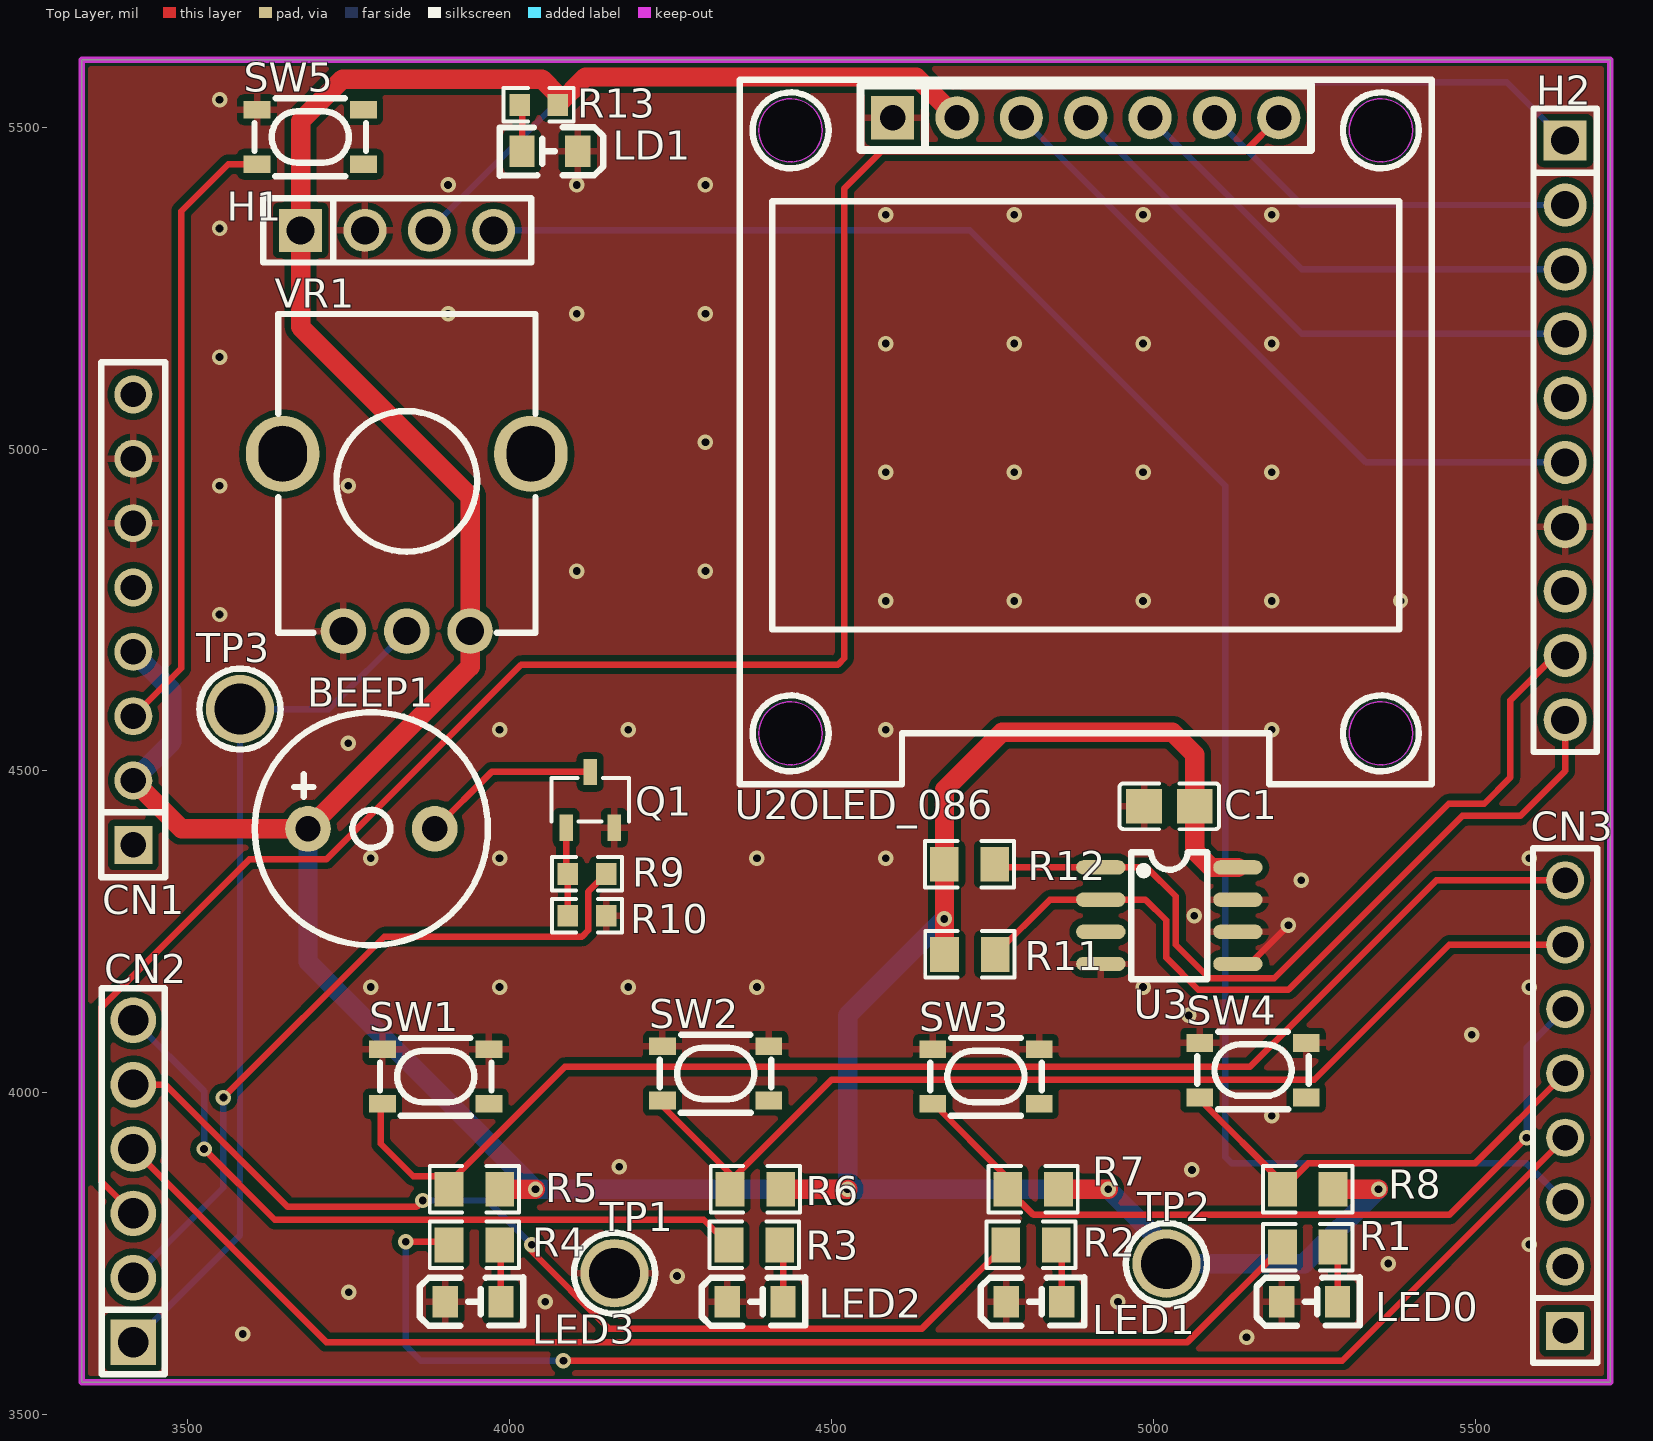
[diagram p0: Top Layer view]
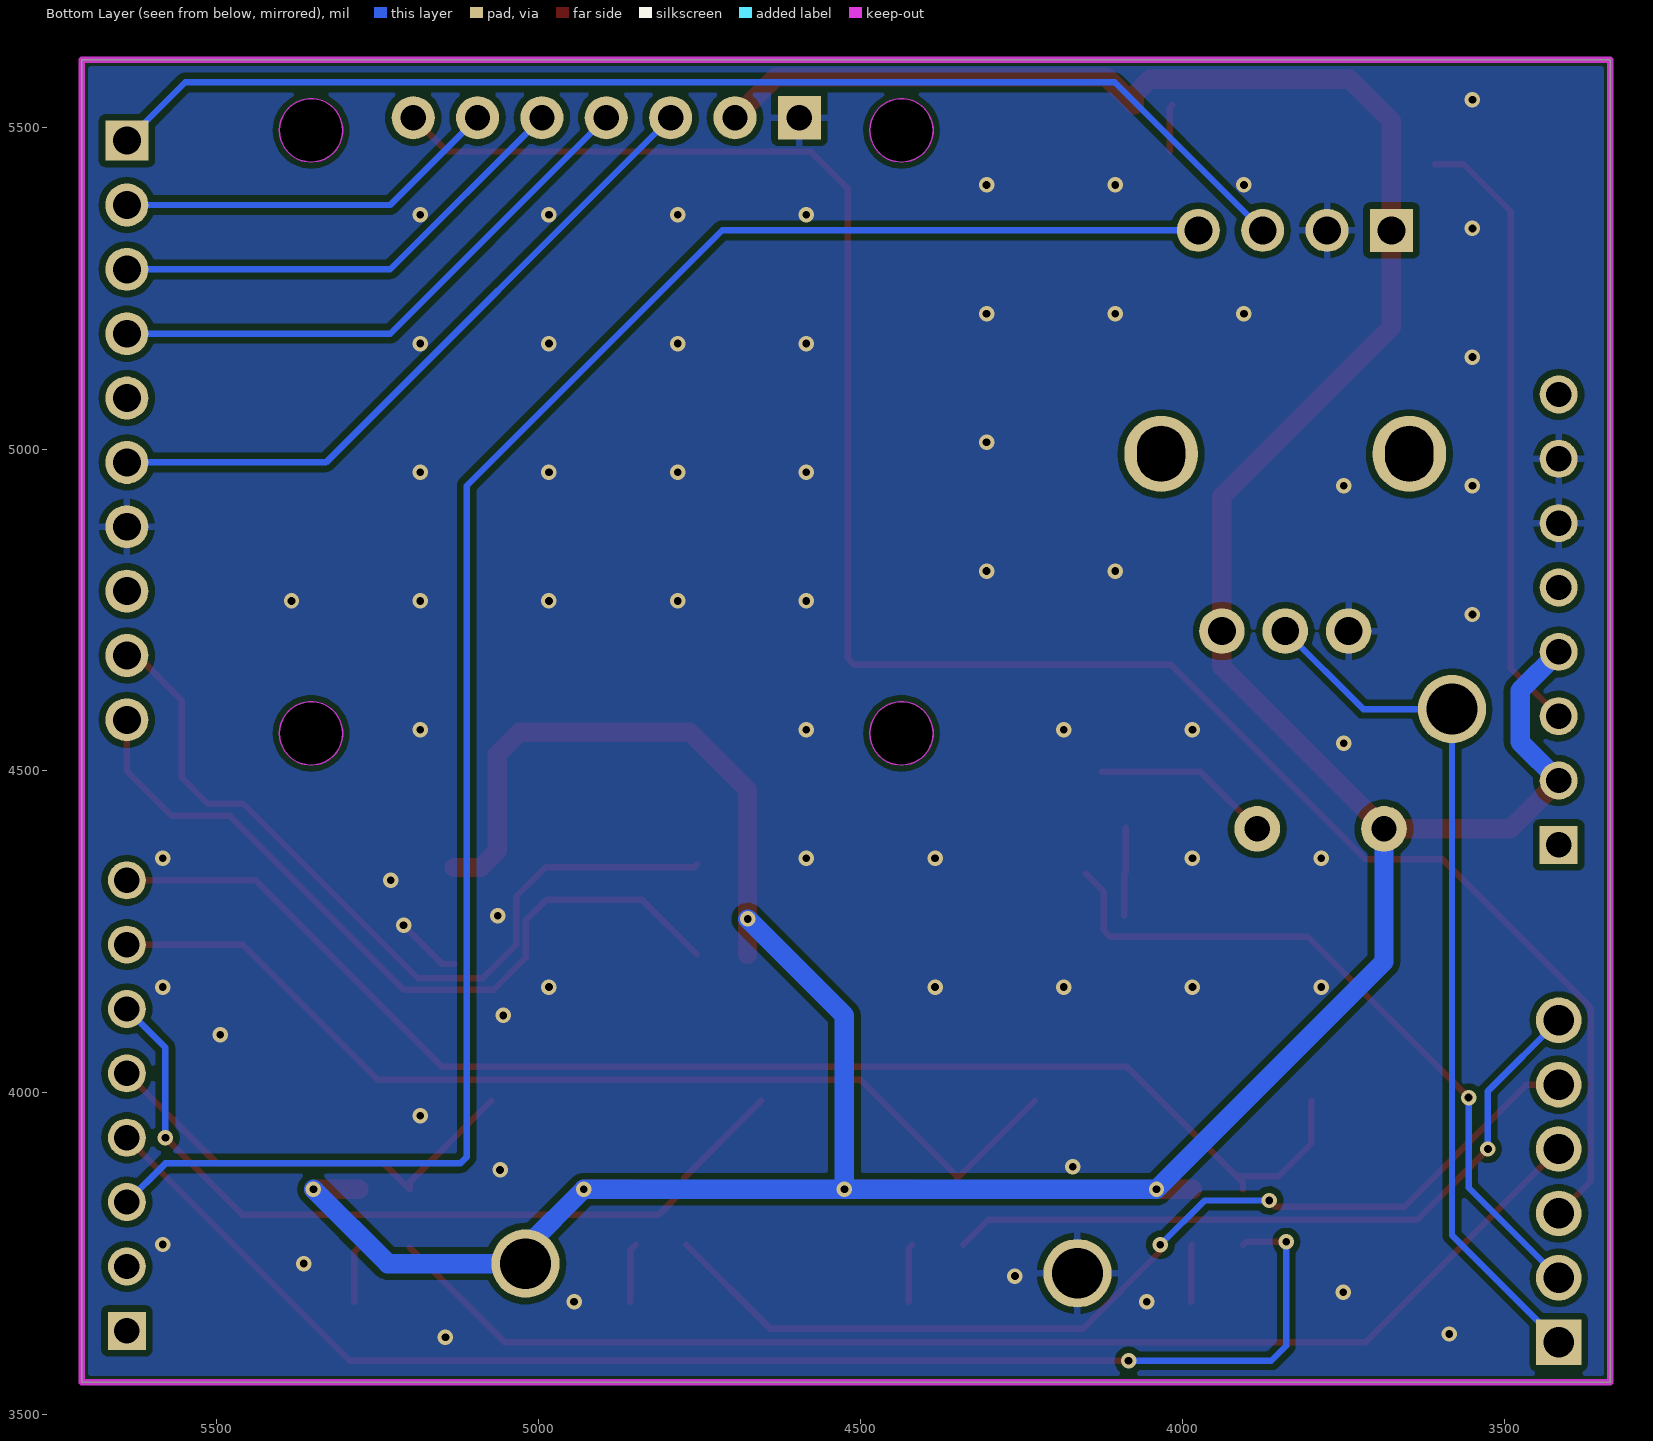
[diagram p1: Bottom Layer view, seen from below]
# Altium PCB MISC51904.pcbdoc
Units mil, origin at the board's own origin, x right, y up, seen from the top; angles counter-clockwise.
Board outline 2375 x 2055 mil, 2 copper layers (Top Layer, Bottom Layer), stack 62.206 mil thick; 37 components, 32 nets, 122 pads, 76 vias.

## Layer stack, top to bottom
Top Solder Mask Layer: solder mask 0.394, Dk 3.3
Top Layer: signal copper 1.379
Dielectric1: surface 59.449, FR4, Dk 4.5
Bottom Layer: signal copper 1.378
Bottom Solder Mask Layer: solder mask 0.394, Dk 3.3

## Board outline
3335,5605 3335,3550 5710,3550 5710,5605

## Design rules (kind name [scope] priority, off if disabled: settings)
BoardOutlineClearance copperThickness2oz_1 [All] p2 off: genericclearance=7.99 ignorepadtopadclearanceinfootprint=FALSE except(0: Arc-SplitContinuation Track-SplitContinuation SMDPad-SplitContinuation THPad-SplitContinuation Via-SplitContinuation Fill-SplitContinuation Region-SplitContinuation Poly-SplitContinuation Text-SplitContinuation Hole-SplitContinuation; 5.98: Arc-CutoutEdge SMDPad-CutoutEdge THPad-CutoutEdge Via-CutoutEdge Fill-CutoutEdge Region-CutoutEdge Text-CutoutEdge; 6.93: Hole-OutlineEdge Hole-CutoutEdge; 10: Poly-OutlineEdge Poly-CutoutEdge; 11.81: Arc-OutlineEdge Track-OutlineEdge SMDPad-OutlineEdge THPad-OutlineEdge Via-OutlineEdge Fill-OutlineEdge Region-OutlineEdge Text-OutlineEdge Track-CutoutEdge)
BoardOutlineClearance copperThickness1oz_1 [All] p4: genericclearance=4.02 ignorepadtopadclearanceinfootprint=FALSE except(0: Arc-SplitContinuation Track-SplitContinuation SMDPad-SplitContinuation THPad-SplitContinuation Via-SplitContinuation Fill-SplitContinuation Region-SplitContinuation Poly-SplitContinuation Text-SplitContinuation Hole-SplitContinuation; 6: SMDPad-CutoutEdge THPad-CutoutEdge Via-CutoutEdge Fill-CutoutEdge Region-CutoutEdge Text-CutoutEdge; 6.93: Hole-OutlineEdge Hole-CutoutEdge; 10: Poly-OutlineEdge Poly-CutoutEdge; 11.8: Arc-OutlineEdge Track-OutlineEdge SMDPad-OutlineEdge THPad-OutlineEdge Via-OutlineEdge Fill-OutlineEdge Region-OutlineEdge Text-OutlineEdge; 11.81: Arc-CutoutEdge Track-CutoutEdge)
Clearance copperThickness2oz [All] p1 off: gap=7.99 ignorepadtopadclearanceinfootprint=FALSE except(5.98: SMDPad-Track SMDPad-SMDPad THPad-Track SMDPad-THPad THPad-THPad Track-Via SMDPad-Via THPad-Via Via-Via Fill-Track Region-Track Fill-SMDPad Region-SMDPad Fill-THPad Region-THPad Fill-Via Region-Via Fill-Fill Fill-Region Region-Region Arc-Track Arc-SMDPad Arc-THPad Arc-Via Fill-Arc Region-Arc Arc-Arc Text-Track SMDPad-Text Text-THPad Text-Via Fill-Text Region-Text Arc-Text Text-Text; 6.93: Hole-Track Hole-SMDPad Hole-THPad Hole-Via Fill-Hole Region-Hole Hole-Arc Hole-Text; 10: Poly-Track Poly-SMDPad Poly-THPad Poly-Via Poly-Fill Poly-Region Poly-Poly Poly-Arc Poly-Text Poly-Hole)
Clearance copperThickness1oz [All] p3: gap=4.02 ignorepadtopadclearanceinfootprint=FALSE except(5.98: SMDPad-Track SMDPad-SMDPad THPad-Track SMDPad-THPad THPad-THPad Track-Via SMDPad-Via THPad-Via Via-Via Fill-Track Region-Track Fill-SMDPad Region-SMDPad Fill-THPad Region-THPad Fill-Via Region-Via Fill-Fill Fill-Region Region-Region; 6: Arc-Track Arc-SMDPad Arc-THPad Arc-Via Fill-Arc Region-Arc Arc-Arc Text-Track SMDPad-Text Text-THPad Text-Via Fill-Text Region-Text Arc-Text Text-Text; 6.93: Hole-Track Hole-SMDPad Hole-THPad Hole-Via Fill-Hole Region-Hole Hole-Arc Hole-Text; 10: Poly-Track Poly-SMDPad Poly-THPad Poly-Via Poly-Fill Poly-Region Poly-Poly Poly-Arc Poly-Text Poly-Hole)
DiffPairsRouting differentialPair [All] p1: maxlimit=6 minlimit=6 mostfreqgap=6 toplayer_minwidth=5 toplayer_prefwidth=10 toplayer_maxwidth=100 toplayer_mingap=6 toplayer_prefgap=6 toplayer_maxgap=6 bottomlayer_minwidth=5 bottomlayer_prefwidth=10 bottomlayer_maxwidth=100 bottomlayer_mingap=6 bottomlayer_prefgap=6 bottomlayer_maxgap=6 maxuncoupledlength=10
HoleToHoleClearance otherClearance [All] p1: gap=11.81 allowstackedmicrovias=TRUE
Length netLength [All] p1: minlimit=0 maxlimit=0
MatchedLengths netLengthTolerance [All] p1: tolerance=1000
PasteMaskExpansion pasteMaskExpansion [All] p1: expansion=0
PlaneConnect innerPlane [All] p1: planeconnectstyle=Relief reliefexpansion=20 reliefentries=4 reliefconductorwidth=10 reliefairgap=10
PolygonConnect copperRegion [(InNet('GND'))] p1: connectstyle=Relief reliefconductorwidth=10 reliefentries=4 polygonreliefangle="90 Angle" airgapwidth=10 via.connectstyle=Relief via.reliefconductorwidth=10 via.reliefentries=4 via.polygonreliefangle="90 Angle" via.airgapwidth=10
RoutingVias viaSize [All] p1: holewidth=12.01 width=24.02 viastyle="Through Hole" minholewidth=11.81 minwidth=19.68 maxholewidth=248.03 maxwidth=393.7
SolderMaskExpansion solderMaskExpansion [IsVia] p1: expansion=-1000 istentingtop=TRUE
SolderMaskExpansion solderMaskExpansion [All] p2: expansion=2 istentingtop=FALSE
Width copperThickness2oz_2 [All] p1 off: maxlimit=100 minlimit=8 preferedwidth=10
Width copperThickness1oz_2 [All] p2: maxlimit=100 minlimit=5 preferedwidth=10

## Components (designator, comment, footprint, x,y, rotation, side; value= is the part's Value field where it differs from the comment)
BEEP1 "3kHz" BUZ-TH_BD9.0-P5.00-D0.6-FD 3785,4410 r0 top
C1 "100nF" C0805 5025,4445 r180 top
CN1 "" HDR-TH_8P-P2.54-V-M 3415,4735 r90 top
CN2 "" HDR-TH_6P-P2.54-V-M-1 3415.02,3862.46 r90 top
CN3 "" HDR-TH_8P-P2.54-V-M 5640,3980 r90 top
H1 "" HDR-TH_4P-P2.54-V-F 3825,5340 r0 top
H2 "" HDR-TH_10P-P2.54-V-M-1 5640,5029.37 r270 top
LD1 "NCD0805R1" LED0805-RD 4062.44,5462.83 r180 top
LED0 "" LED_0805 5245,3675 r0 top
LED1 "" LED_0805 4816.67,3675 r0 top
LED2 "" LED_0805 4383.33,3675 r0 top
LED3 "" LED_0805 3945,3675 r0 top
Q1 "S8050 J3Y(RANGE:200-350)" SOT-23-3_L3.0-W1.7-P0.95-LS2.9-BR 4125,4455 r270 top
R1 "4.7K" R0805 5240,3760 r0 top
R2 "4.7K" R0805 4810,3763.48 r0 top
R3 "4.7K" R0805 4380,3763.48 r0 top
R4 "4.7K" R0805 3945,3763.48 r0 top
R5 "4.7kΩ" R0805 3945,3850 r0 top
R6 "4.7kΩ" R0805 4381.67,3850 r0 top
R7 "4.7kΩ" R0805 4813.33,3850 r0 top
R8 "4.7kΩ" R0805 5240,3850 r0 top
R9 "1K" R0603 4120,4340 r0 top
R10 "10K" R0603 4120,4275 r180 top
R11 "4.7kΩ" R0805 4715,4215 r180 top
R12 "4.7kΩ" R0805 4714.45,4354.91 r0 top
R13 "4.7K" R0603 4045,5535 r0 top
SW1 "" Key_SMD_4.2x3.2x2.5 3885,4025 r0 top
SW2 "" Key_SMD_4.2x3.2x2.5 4320,4030 r0 top
SW3 "" Key_SMD_4.2x3.2x2.5 4740,4025 r0 top
SW4 "" Key_SMD_4.2x3.2x2.5 5155,4035 r0 top
SW5 "" Key_SMD_4.2x3.2x2.5 3690,5485 r0 top
TP1 "TP-红色测试点" TESTPOINT-TH_BD3.2 4162.83,3719.39 r0 top
TP2 "TP-红色测试点" TESTPOINT-TH_BD3.2 5020.52,3734.39 r0 top
TP3 "TP-红色测试点" TESTPOINT-TH_BD3.2 3580.83,4596.07 r0 top
U2OLED_086 "0.96寸OLED_7P" OLED-TH_HS96L01W4S03 4895,5515 r0 top
U3 "LM75AD,118" SOIC-8_L5.0-W4.0-P1.27-LS6.0-BL 5025,4275 r270 top
VR1 "10kΩ" RES-ADJ-TH_RK09K1130AJ3 3840,4855 r0 top

## Footprints (in the part's own frame and the unit in brackets; to place one, negate y for a bottom-side part, rotate by r counter-clockwise, add the part's x,y. Pads: shape width x height; smd on the part's side, far side on the other; paste and mask are expansions set on the pad)
BUZ-TH_BD9.0-P5.00-D0.6-FD [mm]
  round 1.8 hole 1 copper offset 0,0: 1(-2.5,0)
  round 1.8 hole 1: 2(2.5,0)
  silkscreen extent -4.6,-4.6 4.6,4.6
C0805 [mm]
  rect 1.41x1.35 smd paste-100 mask+0.051: 1(-1,0) 2(1,0)
  silkscreen extent -1.96,-0.9 1.96,0.9
HDR-TH_4P-P2.54-V-F [mm]
  rect 1.7x1.7 hole 1.1: 1(-3.81,0)
  round 1.7 hole 1.1: 2(-1.27,0) 3(1.27,0) 4(3.81,0)
  silkscreen extent -5.29,-1.27 5.29,1.27
HDR-TH_6P-P2.54-V-M-1 [mm]
  rect 1.8x1.8 hole 1.2: 1(-6.35,0)
  round 1.8 hole 1.2: 2(-3.81,0) 3(-1.27,0) 4(1.27,0) 5(3.81,0) 6(6.35,0)
  silkscreen extent -7.62,-1.25 7.62,1.25
HDR-TH_8P-P2.54-V-M [mm]
  rect 1.5x1.5 hole 1: 1(-8.89,0)
  round 1.5 hole 1: 2(-6.35,0) 3(-3.81,0) 4(-1.27,0) 5(1.27,0) 6(3.81,0) 7(6.35,0) 8(8.89,0)
  silkscreen extent -10.16,-1.27 10.16,1.27
HDR-TH_10P-P2.54-V-M-1 [mm]
  rect 1.575x1.7 hole 1.1: 1(-11.43,0)
  round 1.7 hole 1.1: 2(-8.89,0) 3(-6.35,0) 4(-3.81,0) 5(-1.27,0) 6(1.27,0) 7(3.81,0) 8(6.35,0) 9(8.89,0) 10(11.43,0)
  silkscreen extent -12.7,-1.25 12.7,1.25
Key_SMD_4.2x3.2x2.5 [mil]
  rect 41.3x27.6 smd paste+0 mask+2: 1(-82.7,42.3) 2(82.7,42.3) 3(-82.7,-42.3) 4(82.7,-42.3)
  silkscreen extent -87,-61 87,60
LED0805-RD [mm]
  rect 1x1.25 smd: 1(-1.1,0) 2(1.1,0)
  silkscreen extent -2.1,-0.95 1.98,0.96
LED_0805 [mm]
  rect 1x1.25 smd paste+0 mask+0.051: 1(-1.15,0.005) 2(1.05,0.005)
  silkscreen extent -2.15,-0.94 1.93,0.97
OLED-TH_HS96L01W4S03 [mm]
  rect 1.7x1.7 hole 1: 1(-7.62,0)
  round 1.7 hole 1: 2(-5.08,0) 3(-2.54,0) 4(0,0) 5(2.54,0) 6(5.08,0) 7(7.62,0)
  Board Outline Layer circle w0.003: c11.65,-0.5 r1.25
  Board Outline Layer circle w0.003: c-11.65,-0.5 r1.25
  Board Outline Layer circle w0.003: c-11.65,-24.3 r1.25
  Board Outline Layer circle w0.003: c11.65,-24.3 r1.25
  Board Outline Layer region: 12.9,-0.5 12.776,-1.042 12.429,-1.477 11.928,-1.719 11.372,-1.719 10.871,-1.477 10.524,-1.042 10.4,-0.5 10.4,-0.5 10.524,0.042 10.871,0.477 11.372,0.719 11.928,0.719 12.429,0.477 12.776,0.042 12.9,-0.5
  Board Outline Layer region: 12.9,-0.5 12.89,-0.657 12.861,-0.811 12.812,-0.96 12.745,-1.102 12.661,-1.235 12.561,-1.356 12.447,-1.463 12.32,-1.555 12.182,-1.631 12.036,-1.689 11.884,-1.728 11.728,-1.747 11.571,-1.747 11.416,-1.728 11.264,-1.689 11.118,-1.631 10.98,-1.555 10.853,-1.463 10.739,-1.356 10.639,-1.235 10.555,-1.102 10.488,-0.96 10.439,-0.811 10.41,-0.657 10.4,-0.5 10.41,-0.343 10.439,-0.189 10.488,-0.04 10.555,0.102 10.639,0.235 10.739,0.356 10.853,0.463 10.98,0.556 11.118,0.631 11.264,0.689 11.416,0.728 11.571,0.748 11.728,0.748 11.884,0.728 12.036,0.689 12.182,0.631 12.32,0.556 12.447,0.463 12.561,0.356 12.661,0.235 12.745,0.102 12.812,-0.04 12.861,-0.189 12.89,-0.343
  Board Outline Layer region: -10.4,-0.5 -10.524,-1.042 -10.871,-1.477 -11.372,-1.719 -11.928,-1.719 -12.429,-1.477 -12.776,-1.042 -12.9,-0.5 -12.9,-0.5 -12.776,0.042 -12.429,0.477 -11.928,0.719 -11.372,0.719 -10.871,0.477 -10.524,0.042 -10.4,-0.5
  Board Outline Layer region: -10.4,-0.5 -10.41,-0.657 -10.439,-0.811 -10.488,-0.96 -10.555,-1.102 -10.639,-1.235 -10.739,-1.356 -10.853,-1.463 -10.98,-1.555 -11.118,-1.631 -11.264,-1.689 -11.416,-1.728 -11.571,-1.747 -11.728,-1.747 -11.884,-1.728 -12.036,-1.689 -12.182,-1.631 -12.32,-1.555 -12.447,-1.463 -12.561,-1.356 -12.661,-1.235 -12.745,-1.102 -12.812,-0.96 -12.861,-0.811 -12.89,-0.657 -12.9,-0.5 -12.89,-0.343 -12.861,-0.189 -12.812,-0.04 -12.745,0.102 -12.661,0.235 -12.561,0.356 -12.447,0.463 -12.32,0.556 -12.182,0.631 -12.036,0.689 -11.884,0.728 -11.728,0.748 -11.571,0.748 -11.416,0.728 -11.264,0.689 -11.118,0.631 -10.98,0.556 -10.853,0.463 -10.739,0.356 -10.639,0.235 -10.555,0.102 -10.488,-0.04 -10.439,-0.189 -10.41,-0.343
  Board Outline Layer region: -10.4,-24.3 -10.524,-24.842 -10.871,-25.277 -11.372,-25.519 -11.928,-25.519 -12.429,-25.277 -12.776,-24.842 -12.9,-24.3 -12.9,-24.3 -12.776,-23.758 -12.429,-23.323 -11.928,-23.081 -11.372,-23.081 -10.871,-23.323 -10.524,-23.758 -10.4,-24.3
  Board Outline Layer region: -10.4,-24.3 -10.41,-24.457 -10.439,-24.611 -10.488,-24.76 -10.555,-24.902 -10.639,-25.035 -10.739,-25.156 -10.853,-25.263 -10.98,-25.355 -11.118,-25.431 -11.264,-25.489 -11.416,-25.528 -11.571,-25.547 -11.728,-25.547 -11.884,-25.528 -12.036,-25.489 -12.182,-25.431 -12.32,-25.355 -12.447,-25.263 -12.561,-25.156 -12.661,-25.035 -12.745,-24.902 -12.812,-24.76 -12.861,-24.611 -12.89,-24.457 -12.9,-24.3 -12.89,-24.143 -12.861,-23.989 -12.812,-23.84 -12.745,-23.698 -12.661,-23.565 -12.561,-23.444 -12.447,-23.337 -12.32,-23.245 -12.182,-23.169 -12.036,-23.111 -11.884,-23.072 -11.728,-23.052 -11.571,-23.052 -11.416,-23.072 -11.264,-23.111 -11.118,-23.169 -10.98,-23.245 -10.853,-23.337 -10.739,-23.444 -10.639,-23.565 -10.555,-23.698 -10.488,-23.84 -10.439,-23.989 -10.41,-24.143
  Board Outline Layer region: 12.9,-24.3 12.776,-24.842 12.429,-25.277 11.928,-25.519 11.372,-25.519 10.871,-25.277 10.524,-24.842 10.4,-24.3 10.4,-24.3 10.524,-23.758 10.871,-23.323 11.372,-23.081 11.928,-23.081 12.429,-23.323 12.776,-23.758 12.9,-24.3
  Board Outline Layer region: 12.9,-24.3 12.89,-24.457 12.861,-24.611 12.812,-24.76 12.745,-24.902 12.661,-25.035 12.561,-25.156 12.447,-25.263 12.32,-25.355 12.182,-25.431 12.036,-25.489 11.884,-25.528 11.728,-25.547 11.571,-25.547 11.416,-25.528 11.264,-25.489 11.118,-25.431 10.98,-25.355 10.853,-25.263 10.739,-25.156 10.639,-25.035 10.555,-24.902 10.488,-24.76 10.439,-24.611 10.41,-24.457 10.4,-24.3 10.41,-24.143 10.439,-23.989 10.488,-23.84 10.555,-23.698 10.639,-23.565 10.739,-23.444 10.853,-23.337 10.98,-23.245 11.118,-23.169 11.264,-23.111 11.416,-23.072 11.571,-23.052 11.728,-23.052 11.884,-23.072 12.036,-23.111 12.182,-23.169 12.32,-23.245 12.447,-23.337 12.561,-23.444 12.661,-23.565 12.745,-23.698 12.812,-23.84 12.861,-23.989 12.89,-24.143
  Multi-Layer board cut-out: 12.9,-0.5 12.776,-1.042 12.429,-1.477 11.928,-1.719 11.372,-1.719 10.871,-1.477 10.524,-1.042 10.4,-0.5 10.4,-0.5 10.524,0.042 10.871,0.477 11.372,0.719 11.928,0.719 12.429,0.477 12.776,0.042 12.9,-0.5
  Multi-Layer board cut-out: -10.4,-0.5 -10.524,-1.042 -10.871,-1.477 -11.372,-1.719 -11.928,-1.719 -12.429,-1.477 -12.776,-1.042 -12.9,-0.5 -12.9,-0.5 -12.776,0.042 -12.429,0.477 -11.928,0.719 -11.372,0.719 -10.871,0.477 -10.524,0.042 -10.4,-0.5
  Multi-Layer board cut-out: -10.4,-24.3 -10.524,-24.842 -10.871,-25.277 -11.372,-25.519 -11.928,-25.519 -12.429,-25.277 -12.776,-24.842 -12.9,-24.3 -12.9,-24.3 -12.776,-23.758 -12.429,-23.323 -11.928,-23.081 -11.372,-23.081 -10.871,-23.323 -10.524,-23.758 -10.4,-24.3
  Multi-Layer board cut-out: 12.9,-24.3 12.776,-24.842 12.429,-25.277 11.928,-25.519 11.372,-25.519 10.871,-25.277 10.524,-24.842 10.4,-24.3 10.4,-24.3 10.524,-23.758 10.871,-23.323 11.372,-23.081 11.928,-23.081 12.429,-23.323 12.776,-23.758 12.9,-24.3
  silkscreen extent -13.65,-26.3 13.65,1.5
R0603 [mil]
  rect 31.75x34.02 smd paste-3937.01 mask+2: 1(-29.66,0) 2(29.66,0)
  silkscreen extent -55,-26 55,26
R0805 [mm]
  rect 1.133x1.377 smd paste-100 mask+0.051: 1(-1,0) 2(1,0)
  silkscreen extent -1.76,-0.92 1.76,0.92
RES-ADJ-TH_RK09K1130AJ3 [mm]
  round 1.8 hole 1.1: 1(-2.5,-3.5) 2(0,-3.5) 3(2.5,-3.5)
  oval 2.9x3 hole 1.9 slot 2.2 at 90 deg: 4(-4.9,3.5) 5(4.9,3.5)
  silkscreen extent -5.08,-3.56 5.08,9.02
SOIC-8_L5.0-W4.0-P1.27-LS6.0-BL [mil]
  oval 22.38x76.78 smd: 1(-75,-106.5) 2(-25,-106.5) 3(25,-106.5) 4(75,-106.5) 5(75,106.5) 6(25,106.5) 7(-25,106.5) 8(-75,106.5)
  silkscreen extent -98,-59 98,59
SOT-23-3_L3.0-W1.7-P0.95-LS2.9-BR [mil]
  rect 40.85x20.95 smd: 1(43.36,-37.4) 2(43.36,37.4) 3(-43.36,0)
  silkscreen extent -34,-60 34,60
TESTPOINT-TH_BD3.2 [mm]
  round 2.7 hole 2 paste+0 mask+0.05: 1(0,0)
  silkscreen extent -1.6,-1.6 1.6,1.6

## Via types
v1: diameter 24.02, hole 12, Top Layer to Bottom Layer, 76 vias

## Nets (pads, with @x,y where several pads share a name; then routed paths per layer and width w, separated by ;. In a path a pad name is that pad's centre, name@x,y a point inside that pad or via, vN(x,y) a via of type N, cw(c..) or ccw(c..) an arc to the next point about the centre after c; other vN are vias at no path point)
$1N7: LED0.2 R1.2 | length 87.7
  Top Layer w10: R1.2 5286.34,3753.03 LED0.2
$1N9: LED1.2 R2.2 | length 91.9
  Top Layer w10: R2.2 4858.01,3754.84 LED1.2
$1N10: LED2.2 R3.2 | length 90.5
  Top Layer w10: R3.2 4424.67,3758.18 LED2.2
$1N11: LED3.2 R4.2 | length 89.1
  Top Layer w10: R4.2 3986.34,3761.51 LED3.2
$1N39: BEEP1.2 Q1.3 | length 278.2
  Top Layer w10: BEEP1.2 3971.78,4498.36 Q1.3
$1N40: Q1.1 R9.1 R10.2 | length 137.8
  Top Layer w10: Q1.1 4087.6,4342.74 R9.1 R10.2
$1N62: CN1.3 SW5.3 | length 963.7
  Top Layer w10: CN1.3 3489.5,4659.5 3489.5,5369.82 3562.38,5442.7 SW5.3
$1N95: LD1.2 R13.1 | length 73.7
  Top Layer w10: R13.1 4019.13,5531.21 LD1.2
GND: C1.2 CN1.6 CN1.7 H1.2 H2.7 LD1.1 LED0.1 LED1.1 LED2.1 LED3.1 Q1.2 R10.1 SW1.1 SW1.2 SW2.1 SW2.2 SW3.1 SW3.2 SW4.1 SW4.2 SW5.1 TP1.1 U2OLED_086.1 U3.4 U3.5 U3.6 U3.7 VR1.1 | length 103.4
  Top Layer w10: U3.5 5150,4200 v1(5210,4260)
  other v1: 5145,3620 3585,3625 4055,3675 4945,3675 3750,3690 4260,3715 5365.11,3734.39 5584.12,3764.1 5060,3880 4170,3885 5184.12,3964.1 5495,4090 5055,4120 3784.12,4164.1 3984.12,4164.1 4184.12,4164.1 4384.12,4164.1 4984.12,4164.1 5584.12,4164.1 5063.5,4275 5230,4330 3784.12,4364.1 3984.12,4364.1 4384.12,4364.1 4584.12,4364.1 5584.12,4364.1 3749.1,4543.01 3984.12,4564.1 4184.12,4564.1 4584.12,4564.1 5184.12,4564.1 3549.1,4743.01 4584.12,4764.1 4784.12,4764.1 4984.12,4764.1 5184.12,4764.1 5384.12,4764.1 4104.1,4810.56 4304.1,4810.56 3549.1,4943.01 3749.1,4943.01 4584.12,4964.1 4784.12,4964.1 4984.12,4964.1 5184.12,4964.1 4304.1,5010.56 3549.1,5143.01 4584.12,5164.1 4784.12,5164.1 4984.12,5164.1 5184.12,5164.1 3904.1,5210.56 4104.1,5210.56 4304.1,5210.56 3549.1,5343.01 4584.12,5364.1 4784.12,5364.1 4984.12,5364.1 5184.12,5364.1 3904.1,5410.56 4104.1,5410.56 4304.1,5410.56 3549.1,5543.01
PA0: CN2.1 TP3.1 VR1.2 | length 1361.6
  Bottom Layer w10: CN2.1 3580.83,3778.27 TP3.1 3718.87,4596.07 VR1.2
PA1: CN2.2 R9.2 | length 1111.7
  Top Layer w10: v1(3555.02,3992.46) 3805.02,4242.46 4112.12,4242.46 4122.12,4252.46 4122.12,4312.46 R9.2
  Bottom Layer w10: CN2.2 3555.02,3852.46 v1(3555.02,3992.46)
PA2: CN3.2
PA3: CN3.1
PA4: CN2.3 U2OLED_086.7 | length 3171
  Top Layer w10: CN2.3 3365.02,3862.46 3365.02,4132.46 3595.02,4362.46 3715.02,4362.46 4017.56,4665 4510,4665 4520,4675 4520,5405 4577.46,5462.46 5142.45,5462.46 U2OLED_086.7
PA5: H2.6 U2OLED_086.3 | length 1066.9
  Bottom Layer w10: U2OLED_086.3 5330.63,4979.37 H2.6
PA6: H2.5
PA7: H2.4 U2OLED_086.4 | length 884
  Bottom Layer w10: U2OLED_086.4 5230.63,5179.37 H2.4
PA8: CN3.8 R5.1 SW1.3 | length 2143.1
  Top Layer w10: SW1.3@3799.5,3987.51 3799.5,3920.5 3850,3870 R5.1@3915.63,3870 ; R5.1 3905.63,3860 R5.1@3915.63,3870 ; CN3.8 5440,4330 5150,4040 4085.63,4040 R5.1@3915.63,3870
PA9: H1.3 H2.1 | length 1897.8
  Bottom Layer w10: H1.3 4105,5570 5549.37,5570 H2.1
PA10: CN3.3 H1.4 | length 2901.6
  Bottom Layer w10: H1.4 4715,5340 5111.79,4943.21 5111.79,3900 5121.79,3890 5580,3890 CN3.3
PB0: CN2.4 R1.1 | length 1971
  Top Layer w10: CN2.4 3715.02,3612.46 5053.09,3612.46 R1.1
PB3: CN3.4 R4.1 | length 2185.8
  Top Layer w10: v1(3838.35,3768.38) 3900.73,3768.38 R4.1 ; v1(4083.48,3583.48) 5293.48,3583.48 CN3.4
  Bottom Layer w10: v1(3838.35,3768.38) 3838.35,3606.65 3861.52,3583.48 v1(4083.48,3583.48)
PB4: CN3.6 R7.1 SW3.3 | length 1284.4
  Top Layer w10: SW3.3@4653.96,3987.49 4773.96,3867.49 R7.1 4813.96,3810 5460,3810 v1(5580,3930)
  Bottom Layer w10: v1(5580,3930) 5580,4070 CN3.6
PB5: CN3.5 R8.1 SW4.3 | length 704
  Top Layer w10: SW4.3@5073.66,3987.51 5200.63,3860.54 R8.1 5240.63,3890 5500,3890 CN3.5
PB6: H2.3 U2OLED_086.5 | length 742.6
  Bottom Layer w10: U2OLED_086.5 5230.63,5279.37 H2.3
PB8: H2.10 R11.1 U3.2 | length 1232.9
  Top Layer w10: R11.1 4839.37,4300 U3.2 4987.8,4300 5020,4267.8 5020,4210 5070,4160 5210,4160 5480,4430 5570,4430 5640,4500 H2.10
PB9: H2.9 R12.2 U3.1 | length 1281.5
  Top Layer w10: R12.2 4758.74,4350 U3.1 4990,4350 5035,4305 5035,4230 5087.17,4177.83 5187.83,4177.83 5459.06,4449.06 5514.06,4449.06 5555,4490 5555,4610 5624.37,4679.37 H2.9
PB10: CN3.7 R6.1 SW2.3 | length 1631.8
  Top Layer w10: SW2.3@4229.22,3987.51 4346.73,3870 R6.1@4350,3870 ; R6.1 4350,3857.71 R6.1@4350,3870 ; CN3.7 5460,4230 5250,4020 4500,4020 R6.1@4350,3870
PC0: CN2.6 R3.1 | length 1122.9
  Top Layer w10: v1(3525.02,3912.46) 3635.02,3802.46 4301.65,3802.46 R3.1
  Bottom Layer w10: CN2.6 3525.02,4002.46 v1(3525.02,3912.46)
PC1: CN2.5 R2.1 | length 1580.6
  Top Layer w10: CN2.5 3465.02,4012.46 3655.02,3822.46 3855.02,3822.46 v1(3865.02,3832.46) ; v1(4034,3763.48) 4034,3753.48 4154,3633.48 4640.63,3633.48 R2.1
  Bottom Layer w10: v1(3865.02,3832.46) 3965.02,3832.46 v1(4034,3763.48)
PC7: H2.2 U2OLED_086.6 | length 601.2
  Bottom Layer w10: U2OLED_086.6 5230.63,5379.37 H2.2
VD33: BEEP1.1 C1.1 CN1.2 CN1.4 H1.1 R5.2 R6.2 R7.2 R8.2 R11.2 R12.1 R13.2 TP2.1 U2OLED_086.2 U3.8 VR1.3 | length 6822.2
  Top Layer w30: CN1.2 3490,4410 BEEP1.1 3938.42,4661.85 VR1.3 3938.42,4926.58 3675,5190 H1.1 3675,5510 3740,5575 4050,5575 4074.66,5550.34 R13.2 4117.86,5578.2 4631.8,5578.2 U2OLED_086.2 ; R5.2 v1(4040,3850) ; R6.2 v1(4525,3850) ; R11.2 4675.63,4470.63 4765,4560 5030,4560 5064.37,4525.63 C1.1 5064.37,4375.63 5090,4350 U3.8 ; R7.2 v1(4930,3850) ; R8.2 v1(5350,3850)
  Bottom Layer w30: CN1.2 3475,4545 3475,4625 CN1.4 ; BEEP1.1 3686.57,4203.43 v1(4040,3850) v1(4525,3850) ; v1(4675,4270) 4525,4120 v1(4525,3850) ; v1(5350,3850) 5234.39,3734.39 TP2.1 5020.52,3759.48 v1(4930,3850) v1(4525,3850)
pads on no net: CN1.1 CN1.5 CN1.8 H2.8 SW1.4 SW2.4 SW3.4 SW4.4 SW5.2 SW5.4 U3.3 VR1.4 VR1.5

## Polygon pours and split planes (outlines as drawn)
GND on Bottom Layer (solid, remove dead copper, pour order 2): 3000,5860 3000,3000 6180,3000 6180,5860
GND on Top Layer (solid, remove dead copper, pour order 0): 3035,5795 3035,3117.3 5889.84,3117.3 5889.84,5795

## Keep-outs
Board Outline Layer:
  the board outline again, w10